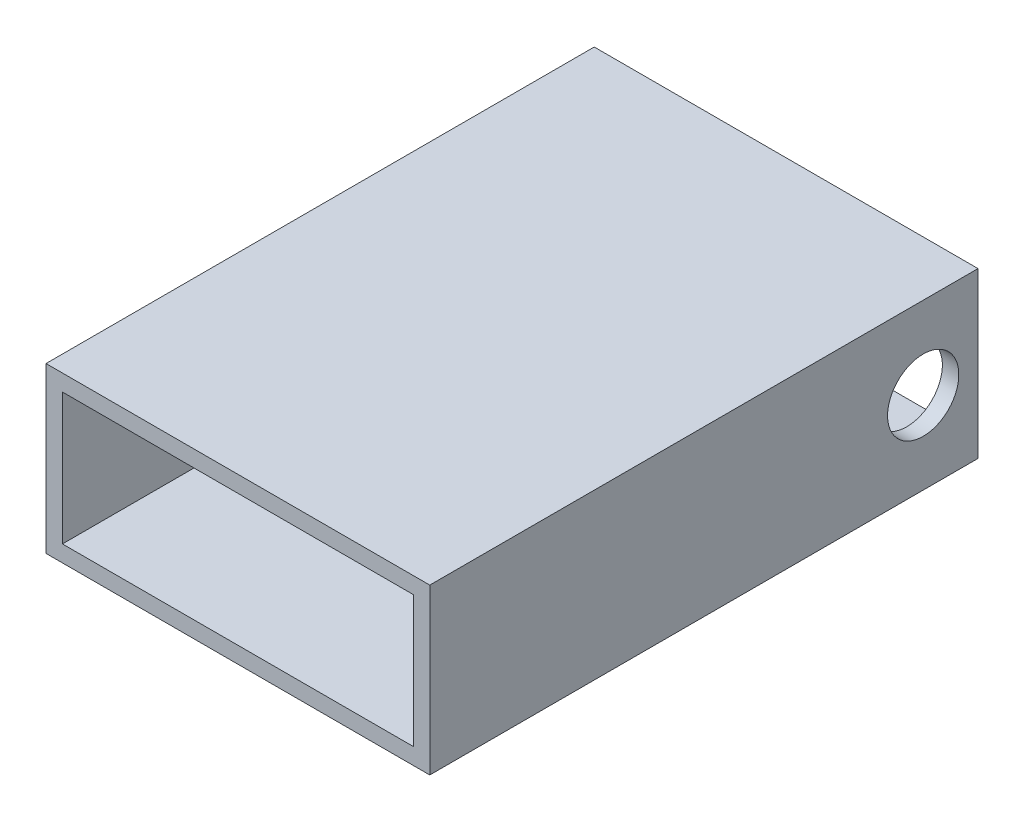
from build123d import *

# Parameters (mm, degrees)
SKETCH_1_W          = 70
SKETCH_1_H          = 30
EXTRUDE_1_DEPTH     = 100
SHELL_1_T           = -3
SKETCH_2_R          = 6.5
CUT_EXTRUDE_2_DEPTH = 100


with BuildPart() as part:
    # 草图1 → 凸台-拉伸1 (new body)
    with BuildSketch(Plane.XY):
        with Locations((35, 15)):
            Rectangle(SKETCH_1_W, SKETCH_1_H)
    extrude(amount=EXTRUDE_1_DEPTH)

    # 抽壳1
    shell_1_openings = [part.faces().sort_by_distance(p)[0] for p in [
        (35, 15, 100),
        (35, 15, 0),
    ]]
    offset(amount=SHELL_1_T, openings=shell_1_openings, kind=Kind.INTERSECTION)

    # 草图2 → 切除-拉伸2 (cut)
    with BuildSketch(Plane.ZY):
        with Locations((10, 15)):
            Circle(SKETCH_2_R)
    extrude(amount=-CUT_EXTRUDE_2_DEPTH, mode=Mode.SUBTRACT)


solid = part.part
